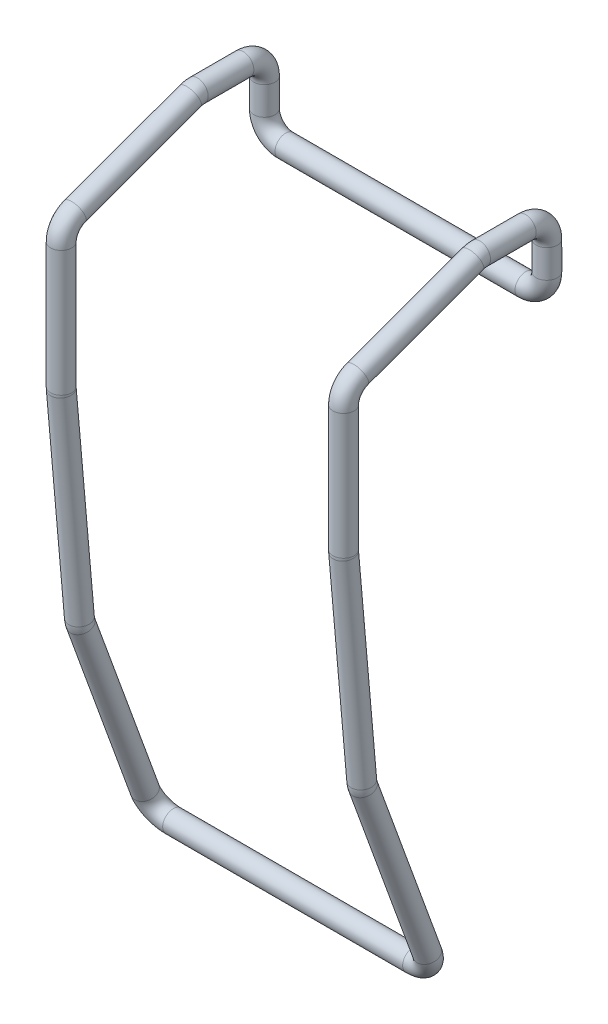
from build123d import *

# Parameters (mm, degrees)
SKETCH1_R = 1.5


with BuildPart() as part:
    # Sweep1: sweep along a curve in space
    with BuildLine() as sweep1_path:
        Line((0, 0, 0), (17, 0, 0))
        ThreePointArc((20, 2.819077862, 1.02606043), (19.121320344, 0.825688789, 0.300526142), (17, 0, 0))
        Line((20, 2.819077862, 1.02606043), (20, 27.819639982, 10.125520881))
        ThreePointArc((20, 28.584233184, 10.295027113), (20, 28.19638157, 10.23533104), (20, 27.819639982, 10.125520881))
        Line((20, 28.584233184, 10.295027113), (20, 57.946135167, 12.863860676))
        ThreePointArc((20, 58.207602395, 12.875276582), (20, 58.076744233, 12.872421247), (20, 57.946135167, 12.863860676))
        Line((20, 58.207602395, 12.875276582), (20, 75.975996952, 12.875276582))
        ThreePointArc((20, 75.975996952, 12.875276582), (20, 77.696726261, 12.332732715), (20, 78.795074814, 10.901337012))
        Line((20, 78.795074814, 10.901337012), (20, 84.736100295, -5.421496346))
        ThreePointArc((20, 84.917022433, -6.447556776), (20, 84.871445692, -5.926612243), (20, 84.736100295, -5.421496346))
        Line((20, 84.917022433, -6.447556776), (20, 84.917022433, -12.918575834))
        ThreePointArc((20, 81.917022433, -15.918575834), (20, 84.038342776, -15.039896177), (20, 84.917022433, -12.918575834))
        Line((20, 81.917022433, -15.918575834), (20, 77.917022433, -15.918575834))
        ThreePointArc((17, 74.917022433, -15.918575834), (19.121320343, 75.795702089, -15.918575834), (20, 77.917022433, -15.918575834))
        Line((17, 74.917022433, -15.918575834), (0, 74.917022433, -15.918575834))
    # Sketch1 → Sweep1 (sweep)
    with BuildSketch(Plane(origin=(0, 0, 0), x_dir=(0, 0, -1), z_dir=(1, 0, 0))):
        Circle(SKETCH1_R)
    sweep1 = sweep(path=sweep1_path.line)

    # Mirror1: Sweep1 across plane
    add(sweep1.mirror(Plane(origin=(0, 74.917022433, -15.918575834), x_dir=(0, 0, 1), z_dir=(-1, 0, 0))))


solid = part.part
